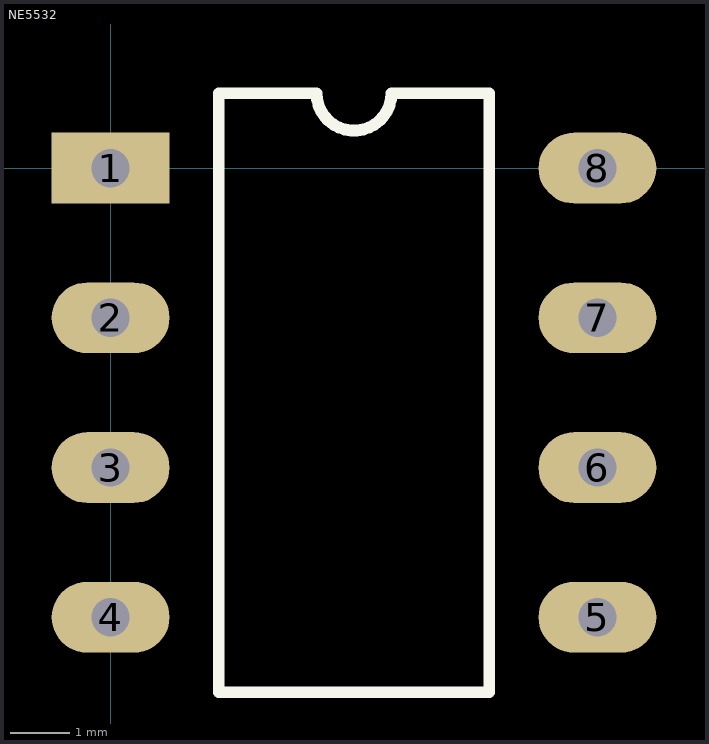
[diagram p0: the footprints below, top view; thin cyan lines are the x and y axes]
# Altium footprint library MISC89340-11.PcbLib: 2 footprints
Each footprint in its own frame and in the unit in brackets; x right, y up, seen from the top. Pads: shape width x height; smd on the part's side, far side on the other; paste and mask are expansions set on the pad; w line width, h text height; cw(c..) or ccw(c..) is an arc to the next point about the centre after c.

## NE5532 [mm]
pads (8):
  rect 2x1.2 hole 0.65: 1(0,0)
  oval 2x1.2 hole 0.65: 2(0,-2.54) 3(0,-5.08) 4(0,-7.62) 5(8.26,-7.62) 6(8.26,-5.08) 7(8.26,-2.54) 8(8.26,0)
Top Overlay:
  lines w0.2: 1.835,-8.89 6.425,-8.89 6.425,1.27 4.765,1.27 cw(c4.13,1.27) 3.495,1.27 1.835,1.27 1.835,-8.89

## PCBComponent_1 [mm]